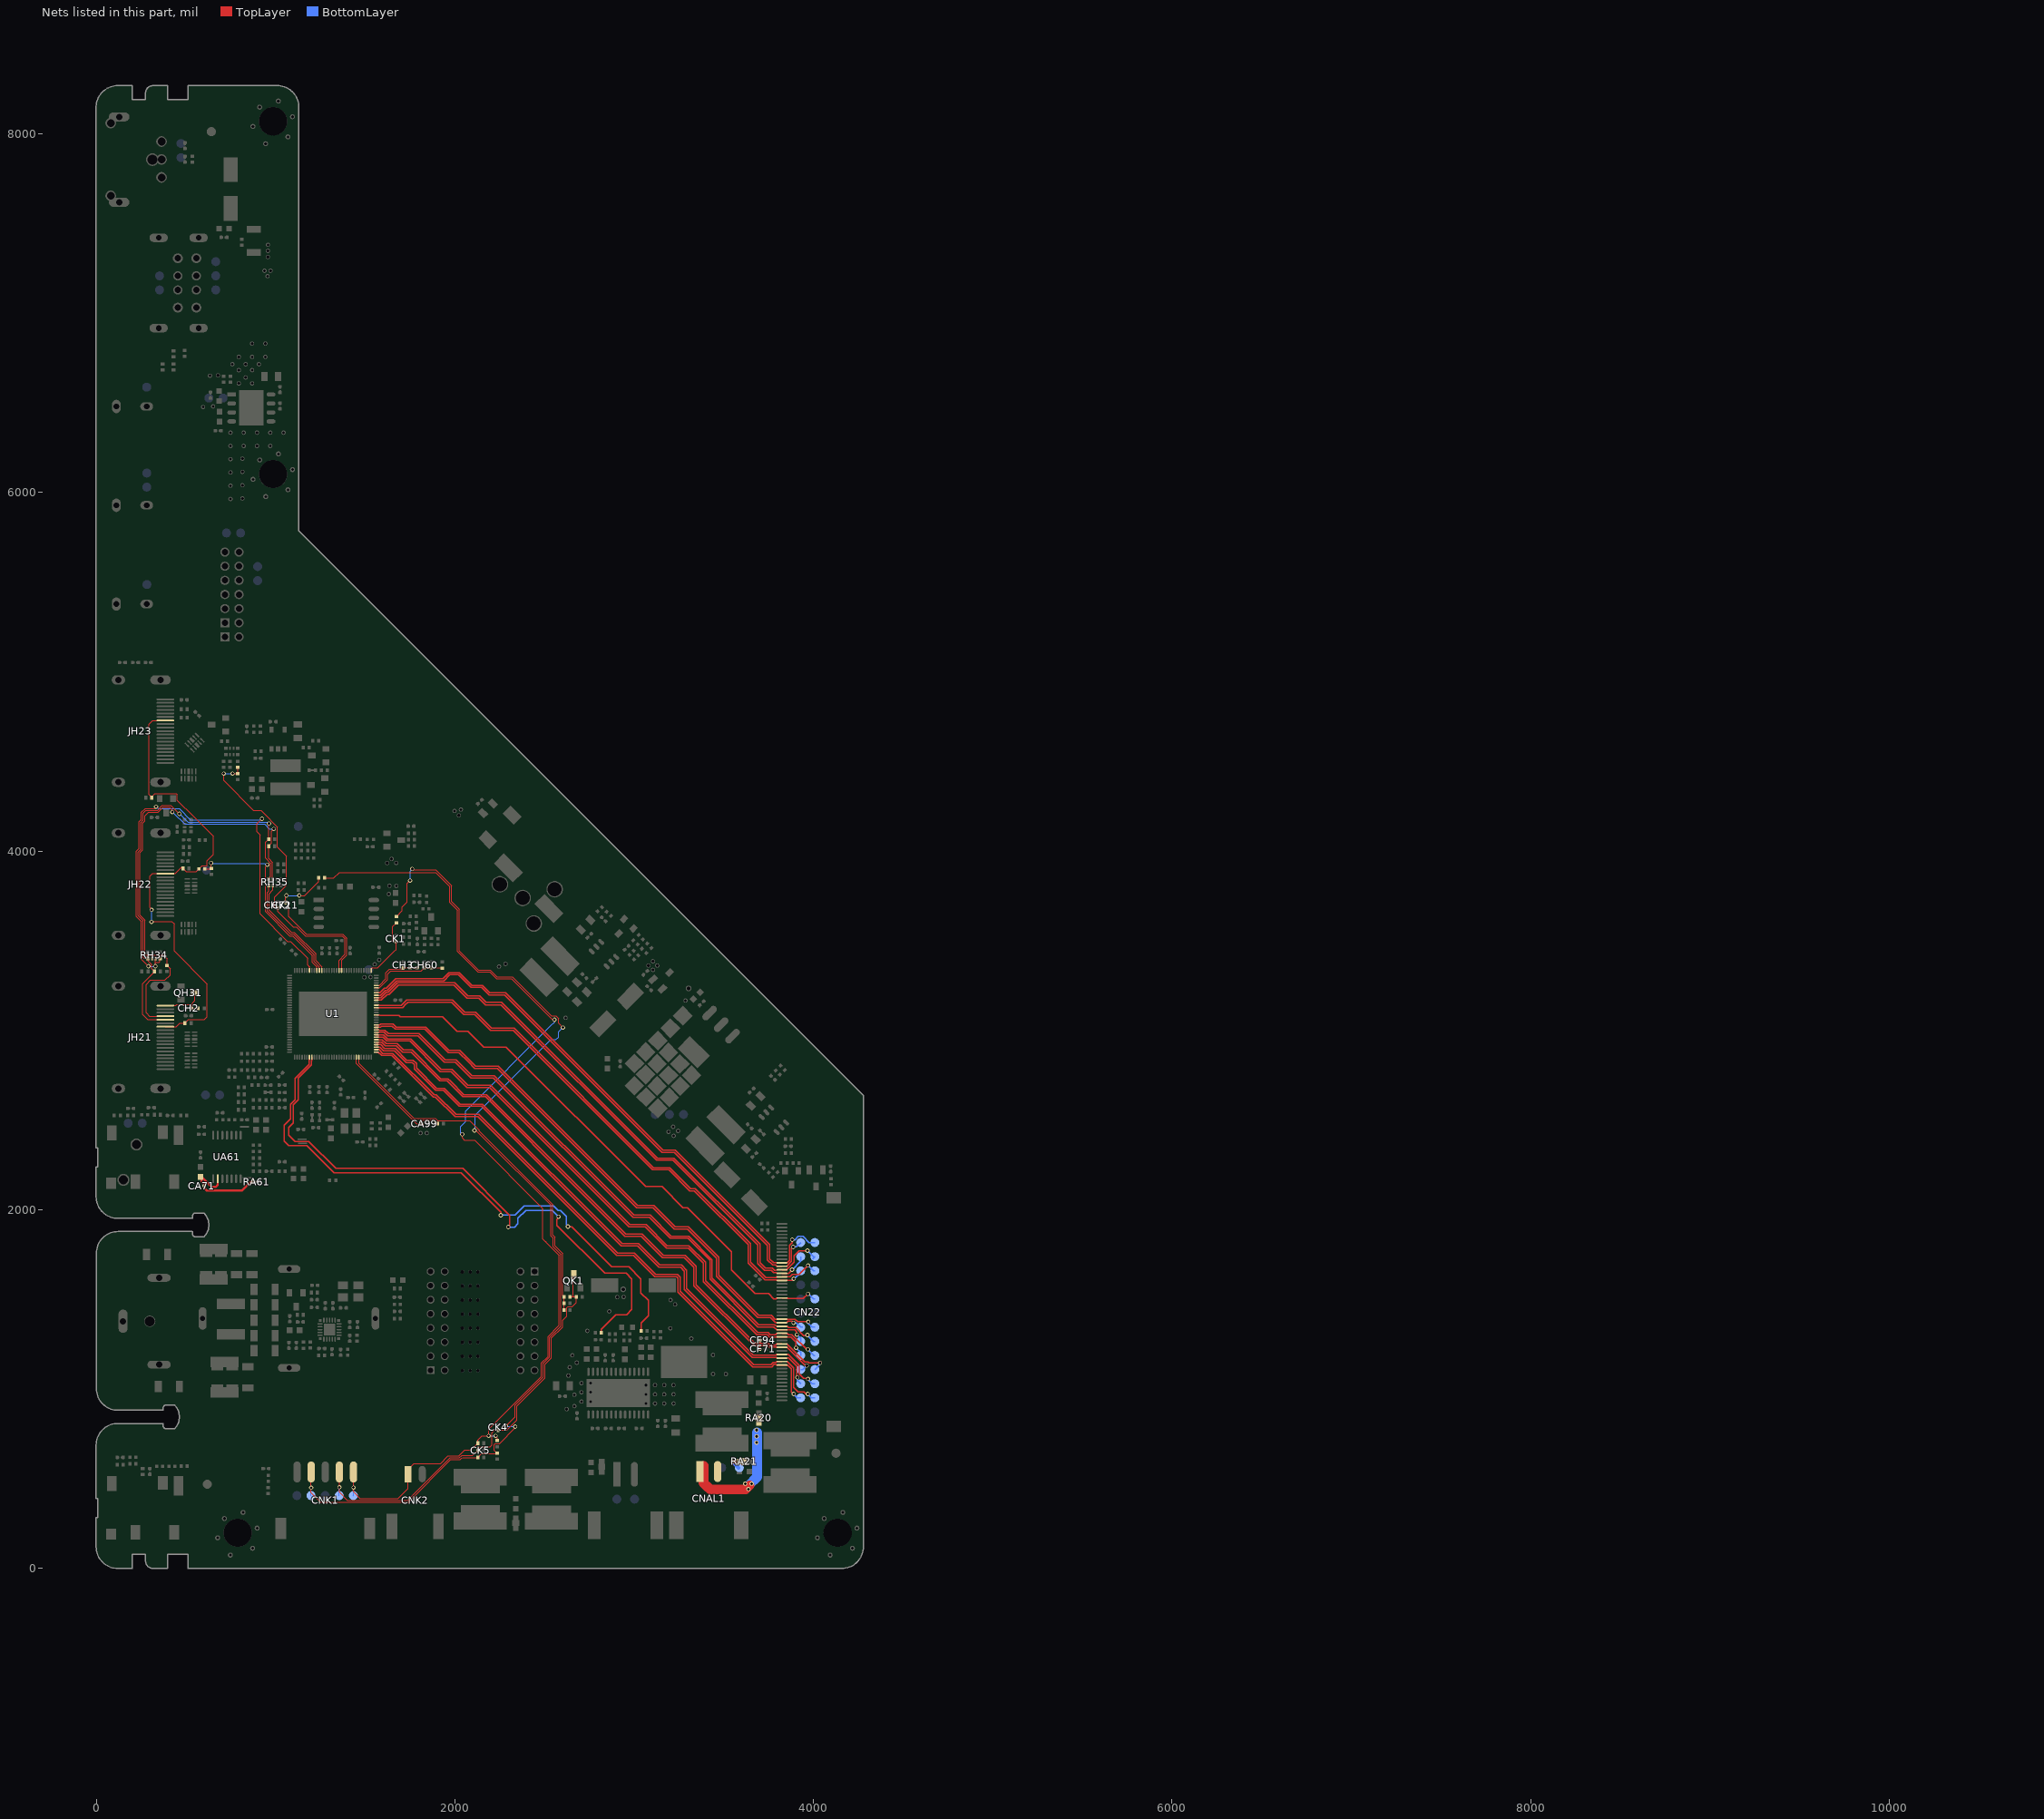
[diagram p0: the nets of this part, all layers, seen from the top]
# Altium PCB MISC105950.PcbDoc (part 11 of 15)
Units mil, origin at the board's own origin, x right, y up, seen from the top; angles counter-clockwise.
Board outline 4280.62 x 8272.76 mil, 2 copper layers (TopLayer, BottomLayer), stack 61.855 mil thick; 541 components, 268 nets, 2324 pads, 1157 vias.

## Via types
v1: diameter 23.62, hole 15.75, TopLayer to BottomLayer, tented both sides, 1087 vias
v2: diameter 23.62, hole 15.75, TopLayer to BottomLayer, 51 vias
v3: diameter 27.56, hole 19.68, TopLayer to BottomLayer, 15 vias
v4: diameter 31.5, hole 19.68, TopLayer to BottomLayer, tented both sides, 4 vias

## Nets (pads, with @x,y where several pads share a name; then routed paths per layer and width w, separated by ;. In a path a pad name is that pad's centre, name@x,y a point inside that pad or via, vN(x,y) a via of type N, cw(c..) or ccw(c..) an arc to the next point about the centre after c; other vN are vias at no path point) (continued)
HDMI_C_HPD_OUT: CH2.1 JH21.19 QH31.C RH33.1 | length 328.2
  TopLayer w5: JH21.19@384.7,3137.25 JH21.19@384.16,3137.8 ; JH21.19@429.3,3137.8 JH21.19@384.16,3137.8 ; 527.65,3142.58 524.92,3142.58 ; QH31.C@549.03,3208 549.03,3166.69 529.23,3146.89 ; RH33.1@566.77,3123 CH2.1@529.23,3123 529.23,3146.89 ; JH21.19@384.16,3137.8 442,3137.8 446.78,3142.58 524.92,3142.58 ; 524.92,3142.58 529.23,3146.89
HDMI_C_HPD_OUT_IC: RH34.2 RH34.4 U1.122 | length 2753
  TopLayer w5: v1(289.26,3357.14) 249.5,3396.9 249.5,3606.45 221.5,3634.45 221.5,3998.62 236.5,4013.62 236.5,4163.19 250.31,4177 250.31,4216.86 271.29,4237.84 v1@327.98,4237.84 ; v1(327.88,3357.14) 327.88,3378 ; RH34.4@330.38,3401.07 327.88,3398.57 327.88,3378 ; RH34.2@354,3401.07 354,3385 347,3378 327.88,3378 ; 913,3994 913,3970 ; v1(922.5,4179.5) 896,4153 896,4108.22 913,4091.22 913,3970 ; U1.122@1185.65,3335.98 U1.122@1187.59,3334.04 1187.59,3352.91 1179.82,3360.68 ; 1185.65,3354.85 1179.82,3360.68 ; 913,3970 913,3648.71 1065.4,3496.31 1082.14,3496.31 1177.66,3400.8 1177.66,3362.84 1179.82,3360.68
  BottomLayer w5: v1(289.26,3357.14) v1(327.88,3357.14) ; v1(331.5,4247.5) 342.64,4236.36 460.95,4236.36 522.81,4174.5 v1@917.5,4174.5
HDMI_C_SCL_IN: DH2.K DH73.K JH21.15 RH34.8 RH35.7 | length 2448.4
  TopLayer w5: DH2.K@322.25,3327.48 DH2.K@323.27,3326.46 ; JH21.15@384.16,3059.06 285.44,3059.06 257.5,3087 257.5,3260.69 DH2.K@323.27,3326.46 ; v1(462,4208) 458.42,4208 412.8,4253.62 365.5,4253.62 339.72,4227.84 275.44,4227.84 260.31,4212.72 260.31,4172.86 246.5,4159.05 246.5,4009.47 231.5,3994.47 231.5,3638.59 259.5,3610.59 259.5,3407 265.43,3401.07 RH34.8@287.07,3401.07 287.07,3386.64 308.57,3365.14 308.57,3349.14 308.57,3343.2 DH2.K@323.27,3328.5 DH2.K@323.27,3326.46 ; RH35.7@960.54,3844.22 960.54,3848.01 971.81,3859.28 971.81,3931.5 943,3960.31 943,4048.47 DH73.K@960.04,4065.5 960.04,4152.04 v1(961.5,4153.5)
  BottomLayer w5: v1(462,4208) 509.81,4160.19 951.81,4160.19 958.5,4153.5 v1(961.5,4153.5)
HDMI_C_SCL_IN_IC: RH35.8 U1.118 | length 607.7
  TopLayer w5: RH35.8@960.54,3808.78 960.54,3777.04 953,3769.5 953,3665.28 1081.81,3536.47 1098.55,3536.47 1213.66,3421.37 1213.66,3383.41 1242.71,3354.36 U1.118@1242.71,3334.04
HDMI_C_SDA_IO: DH3.K DH74.K JH21.16 RH34.6 RH35.5 | length 2559.8
  TopLayer w5: RH34.6@310.69,3401.07 310.69,3418.96 ; JH21.16@384.16,3078.74 295.76,3078.74 276.5,3098 276.5,3254.5 301.16,3279.16 382,3279.16 410.83,3307.98 410.83,3342.91 DH3.K@392.5,3361.23 392.5,3399.36 372.7,3419.16 274.12,3419.16 269.5,3423.78 269.5,3614.74 241.5,3642.74 241.5,3990.33 256.5,4005.33 256.5,4154.9 270.31,4168.72 270.31,4196.98 291.17,4217.84 343.87,4217.84 369.65,4243.62 407.35,4243.62 422.06,4228.92 ; 976.39,4090.89 976.39,4083 ; RH35.5@984.16,3844.22 981.81,3846.56 981.81,3935.64 960.04,3957.42 DH74.K@960.04,4027.5 976.39,4043.86 976.39,4083 ; v1(988.5,4123.5) 976.39,4111.39 976.39,4083
  BottomLayer w5: v1@427.82,4214.49 492.12,4150.19 936.93,4150.19 963.62,4123.5 v1(988.5,4123.5)
  other v1: 422.06,4217.05
HDMI_C_SDA_IO_IC: RH35.6 U1.117 | length 614.9
  TopLayer w5: RH35.6@984.16,3808.78 984.16,3783.39 963,3762.24 963,3669.42 1085.95,3546.47 1102.69,3546.47 1222.66,3426.51 1222.66,3388.56 1256.49,3354.72 U1.117@1256.49,3334.04
HDMI_CEC_IO: DH1.K DH21.K DH70.K JH21.13 JH22.13 JH23.13 RH83.2 | length 2770.9
  TopLayer w5: v1(307,3672) 307,3676.5 297.69,3685.81 297.69,3858.69 313.02,3874.02 JH22.13@384.16,3874.02 438.02,3874.02 474.43,3910.43 DH70.K@481.77,3903.1 500.16,3884.71 555.48,3884.71 RH83.2@570.77,3900 588.11,3917.34 613.34,3917.34 617.38,3921.38 617.38,3946.62 651.16,3980.39 651.16,4081.87 549.52,4183.52 544.28,4188.72 ; v1@307.69,3606.7 419.27,3606.7 432.98,3593 432.98,3441.02 616.59,3257.41 616.59,3075.17 600.73,3059.31 512.81,3059.31 DH1.K@493.5,3040 464.42,3040 444.11,3019.69 JH21.13@384.16,3019.69 ; JH23.13@384.16,4728.35 312.85,4728.35 291.71,4707.21 291.71,4316.02 307.23,4300.5 326.42,4319.69 445.35,4319.69 450.61,4314.43 450.61,4282.39 539.85,4193.15 ; 539.88,4193.15 544.28,4188.76
  BottomLayer w5: v1(306,3604.5) v1@307,3605.5 ; v1@310,3608.5 v1@307,3605.5 ; v1@310,3672 v1(307,3672) v1@307,3605.5
HDMI_CEC_IO_IC: DH4.K RH83.1 U1.119 | length 1126.3
  TopLayer w5: RH83.1@604.36,3900.5 DH4.K@648.66,3900.5 ; v1(638.5,3933) 638.5,3904.73 DH4.K@640,3903.23 ; 943,3897.5 943,3885.5 ; v1(952.5,3923.5) 943,3914 943,3885.5 ; U1.119@1228.93,3334.04 1228.93,3353.99 1204.66,3378.27 1204.66,3416.22 1094.41,3526.47 1077.67,3526.47 943,3661.14 943,3885.5
  BottomLayer w5: v1(638.5,3933) 642,3929.5 938,3929.5 944,3923.5 v1(952.5,3923.5)
HDMIA_DET_IC: CH72.2@1011.5,3681.66 CH72.2@1011.5,3688.55 RH74.1 RH75.1 U1.110 | length 1765.6
  TopLayer w5: v1@700.5,4432.5 v1(709.5,4432.5) 709.5,4392.64 875.16,4226.98 916.63,4226.98 929.61,4214 929.82,4214 1009.86,4133.96 1009.86,4020.99 1060.36,3970.49 1060.36,3810.17 993,3742.81 993,3687 998.34,3681.66 CH72.2@1011.5,3681.66 1011.5,3663.35 1098.38,3576.47 1115.12,3576.47 1165.28,3526.31 1369.79,3526.31 1386.66,3509.44 1386.66,3423.98 1352.95,3390.27 U1.110@1352.95,3334.04 ; v1@757.51,4432.49 RH75.1@787.75,4432.49 ; v1@758.51,4432.49 RH75.1@787.75,4432.49 ; RH75.1@784.5,4436.5 RH75.1@787.75,4433.25 ; RH74.1@787.75,4466.53 RH75.1@787.75,4433.25 ; RH75.1@787.75,4432.49 RH75.1@787.75,4433.25
  BottomLayer w5: v1(709.5,4432.5) v1@757.5,4432.5
  other v1: 758.5,4432.5
HDMIB_DET_IC: CH60.2@1828.5,3347.76 CH60.2@1828.5,3354.65 RH1.1 RH2.1 U1.91 | length 467.9
  TopLayer w5: U1.91@1560.66,3236.56 1577.34,3236.56 1623.94,3283.16 1623.94,3289.05 1623.94,3313.33 1641.11,3330.5 1699.05,3330.5 1699.15,3330.4 1719.85,3330.4 1719.95,3330.5 1723,3330.5 1811.24,3330.5 CH60.2@1828.5,3347.76 ; CH60.2@1829,3348.27 CH60.2@1828.5,3347.76 ; RH2.1@1868.5,3347.77 RH1.1@1928.5,3347.77 ; 1904,3347.76 CH60.2@1828.5,3347.76
HDMIC_DET_IC: CH3.2@1709.5,3346.76 CH3.2@1709.5,3353.65 RH81.1 RH82.1 U1.92 | length 299.6
  TopLayer w5: U1.92@1560.66,3250.34 1576.97,3250.34 1613.94,3287.31 1613.94,3320.3 1634.83,3341.19 1697.04,3341.19 CH3.2@1709.5,3353.65 ; CH3.2@1703.24,3340.5 1711.5,3348.77 RH81.1@1786,3348.77 RH81.1@1784.23,3347
HP_DET_IC: CA99.2@1812.61,2478.5 CA99.2@1819.5,2478.5 RA52.2 U1.58 | length 652
  TopLayer w5: U1.58@1449.41,2849.72 1449.41,2813.71 1784.61,2478.5 CA99.2@1812.61,2478.5 1812.61,2492.61 1817.81,2497.81 1882.96,2497.81 RA52.2@1902.27,2478.5
HP_VDD: CA70.1 CA71.1 RA61.2 RA61.3 UA61.9 | length 546
  TopLayer w12: CA70.1@579.5,2189.19 CA70.1@584.5,2189.19 ; CA70.1@584.5,2183.5 642.5,2125.5 664.5,2125.5 676,2137 UA61.9@676,2171.5 ; CA70.1@584.5,2190 584.5,2157.5 601.86,2140.14 601.86,2118.14 614.54,2105.46 810.38,2105.46 844.96,2140.04 ; 850.26,2145.35 844.96,2140.04 ; RA61.2@875.77,2155 859.92,2155 844.96,2140.04
IR: CNK1.2 DK4.K IR.1 RK6.1 RK25.1 | length 6071
  TopLayer w5: CNK1.2@1197.16,535.5 v1(1197.16,447.88) 1197.16,420.34 1249.12,368.38 1739.45,368.38 1976.29,605.21 2028.87,605.21 2035.51,611.86 2040.15,616.5 DK4.K@2127.27,616.5 2147.96,637.19 RK25.1@2238.96,637.19 ; RK6.1@1673.5,3633.73 1673.5,3634.14 1705.68,3666.32 1705.68,3688.32 1732.91,3715.56 1732.91,3819.41 v1(1748.5,3835) ; v1@1761,3894.5 1893.14,3894.5 1981.5,3806.14 1981.5,3716.92 2023.31,3675.11 2023.31,3443.2 2131.01,3335.5 2196.64,3335.5 2234.33,3297.81 2319.55,3297.81 2538.17,3079.19 2563.31,3079.19 2577.5,3065 2577.5,3039 v1(2601.5,3015) ; v1@2117.31,2441 2155.4,2402.9 2534.31,2023.99 2534.31,1853.1 2547,1840.41 2547,1792.32 2590.5,1748.82 2590.5,1349.04 2528.36,1286.91 2528.36,1176.58 2492.36,1140.58 2492.36,1065.29 2335,907.92 2335,844 v1(2283.5,792.5) ; RK25.1@2231.96,637.19 RK25.1@2235.5,640.73 2234.27,640.73 2218.16,656.84 2218.16,689.23 2223.3,694.37 2248.45,694.37 v1@2335.5,781.42
  BottomLayer w5: IR.1@1196.26,403.88 1197.16,404.78 v1(1197.16,447.88) ; v1@1749,3835 1749,3888.5 v1(1761,3900.5) ; v1@2113.17,2445.67 2113.17,2526.57 2534.28,2947.69 2563.5,2947.69 2577.5,2961.69 2577.5,2991 v1(2601.5,3015) ; v1@2287,789 v1(2335.5,789)
  other v1: 2108.5,2441
IR_IN_IC: CK1.2@1670,3494.26 CK1.2@1670,3501.15 RK6.2 U1.97 | length 410.3
  TopLayer w5: U1.97@1532.08,3334.04 1532.08,3344.58 1536.5,3349 1569.1,3349 1661.49,3441.38 1670.47,3450.36 CK1.2@1670.47,3497.8 ; 1652.66,3514.36 1652.66,3529 ; 1652.66,3553.93 1652.66,3529 ; CK1.2@1668.75,3498.26 CK1.2@1670,3498.26 ; CK1.2@1670,3494.26 1657.24,3494.26 1652.66,3498.84 1652.66,3529 ; RK6.2@1673.5,3600.27 1652.66,3579.43 1652.66,3529
K0/AD: CNK1.5 CNK2.1 DK70.K KEY.1 RK2.1 RK23.2 | length 6035.5
  TopLayer w5: RK23.2@1271.73,3850 1323.5,3850 1354.5,3881 1892.5,3881 1971.5,3802 1971.5,3712.78 2013.31,3670.97 2013.31,3439.06 2126.87,3325.5 2167,3325.5 ; CNK1.5@1433.25,535.38 v1(1433.25,449.13) 1433.25,424.75 1469.62,388.38 1681.73,388.38 1737.84,444.48 CNK2.1@1737.84,496.04 ; CNK2.1@1737.84,523.69 1737.84,551.34 1770,583.5 1919,583.5 1960.71,625.21 2020.58,625.21 2053.87,658.5 2088.77,658.5 DK70.K@2127.27,697 2127.27,714.33 2150.44,737.5 v1(2187.5,737.5) 2187.5,774.56 2482.36,1069.43 2482.36,1144.72 2518.36,1180.72 2518.36,1291.05 2580.5,1353.18 2580.5,1744.68 2513.09,1812.09 ; v1(2040,2419.5) 2040,2398.5 2052.5,2386 2108.67,2386 2489.31,2005.35 2489.31,1835.87 2513.09,1812.09 ; 2134.22,3325.5 2167,3325.5 ; v1(2226.5,737.5) 2226.5,733 2235.5,724 RK2.1@2235.5,710.73 ; 2503.2,1821.98 2513.09,1812.09 ; v1(2554.22,3058.57) 2553,3057.35 2553,3050.22 2315.4,3287.81 2230.19,3287.81 2192.5,3325.5 2167,3325.5
  BottomLayer w5: KEY.1@1432.48,403.88 1433.25,404.65 v1(1433.25,449.13) ; v1(2040,2419.5) 2032,2427.5 2032,2463.86 2058.17,2490.02 2058.17,2549.35 2535,3026.19 ; v1(2187.5,737.5) v1(2226.5,737.5) ; 2541,3032.19 2535,3026.19 ; v1(2554.22,3058.57) 2554.22,3045.41 2535,3026.19
KEY_IN_IC: CK11.1 RK23.1 U1.109 | length 953.2
  TopLayer w5: v1(1059.5,3752) 1053.5,3746 CK11.1@1053.5,3716.63 ; v1@1130.07,3754 1128.5,3754 v1(1130.5,3752) 1160.3,3752 1238.27,3829.97 RK23.1@1238.27,3850 ; U1.109@1366.73,3334.04 1368.01,3335.31 1368.01,3391.19 1396.66,3419.84 1396.66,3513.59 1373.93,3536.31 1169.42,3536.31 1117.09,3588.64 1116.88,3588.64 1071,3634.52 1071,3711.5 1067.37,3715.13 CK11.1@1055,3715.13 ; CK11.1@1053.5,3716.63 CK11.1@1053.5,3715.13 CK11.1@1055,3715.13 ; CK11.1@1053.5,3716.63 CK11.1@1055,3715.13
  BottomLayer w5: v1(1059.5,3752) 1086,3752 ; 1098.5,3752 1086,3752 ; v1(1130.5,3752) 1086,3752
LED_R_OUT: CK4.2@2240,767.76 CK4.2@2240,774.65 CK5.2@2126.27,656.5 CK5.2@2133.16,656.5 CNK1.4 LED.1 QK1.C RK10.1 RK14.2 | length 2398
  TopLayer w5: CNK1.4@1354.64,535.5 v1(1354.64,450.24) 1354.64,422.36 1398.62,378.38 1735.31,378.38 1972.14,615.21 2024.72,615.21 2037.4,627.9 2097.66,627.9 CK5.2@2126.27,656.5 2126.27,670.77 2131.31,675.81 2195.24,675.81 2206.81,687.39 2206.81,753.81 2223,770 2289.19,770 2345,825.81 2345,903.78 2502.36,1061.14 2502.36,1136.44 2538.36,1172.44 2538.36,1282.76 2600.5,1344.9 2600.5,1381 2624.37,1404.87 2624.37,1452.95 2630.58,1459.16 2653.2,1459.16 2675.77,1481.73 RK10.1@2675.77,1512.5 2659,1512.5 ; RK14.2@2641.23,1512.5 2659,1512.5 ; QK1.C@2662,1638.03 2659,1635.03 2659,1512.5
  BottomLayer w5: LED.1@1353.74,403.88 v1@1353.74,449.34
LED_R_OUT_IC: RK13.1 RK14.1 RK15.1 U1.59 | length 2060.5
  TopLayer w5: U1.59@1463.19,2849.72 1463.19,2814.07 1769.44,2507.81 1889.53,2507.81 1901.5,2495.84 2080.97,2495.84 2135.31,2441.5 2135.31,2437.14 2544.31,2028.14 2544.31,1858.65 2557,1845.96 2557,1796.47 2600.5,1752.97 2600.5,1519.77 RK14.1@2607.27,1513 ; RK13.1@2607.77,1440.5 RK13.1@2607.27,1440 RK14.1@2607.27,1513 ; RK14.1@2607.77,1512.5 RK14.1@2607.27,1513
LINE_L_OUT_IC: RA3.1 U1.39 | length 3231.6
  TopLayer w7: 1185.82,2830 1185.82,2826 ; U1.39@1187.59,2849.72 1187.59,2835.91 1185.82,2834.13 1185.82,2826 ; v1(2255.15,1968.38) 2255.15,1983.55 2033.69,2205 1325.45,2205 1174.11,2356.34 1072.43,2356.34 1047.69,2381.09 1047.69,2471.19 1082,2505.5 1082,2587 1107,2612 1107,2731.94 1185.82,2810.76 1185.82,2826 ; v1(2629.62,1904.36) 2649.87,1904.36 2873.72,1680.5 2968.75,1680.5 3037,1612.25 3037,1534.56 3078.95,1492.6 3078.95,1408.5 3037.27,1366.81 RA3.1@3037.27,1322
  BottomLayer w7: v1(2255.15,1968.38) 2334.24,1968.38 2385.16,2019.31 2551.13,2019.31 2575.94,1994.5 2588.97,1994.5 2621.31,1962.16 v1@2621.31,1912.67
LINE_R_OUT_IC: RA14.1 U1.40 | length 3338.8
  TopLayer w7: 1134.03,2380.34 1155.5,2380.34 ; U1.40@1200.43,2848.77 U1.40@1201.37,2849.72 1201.37,2832.71 1197.82,2829.16 1197.82,2805.79 1124.5,2732.47 1124.5,2612.53 1096.5,2584.53 1096.5,2482.72 1072.19,2458.41 1072.19,2414.62 1106.46,2380.34 1155.5,2380.34 ; v1@2297.5,1902 v1(2297,1902) 2305.5,1910.5 2305.5,1967.13 2043.63,2229 1335.39,2229 1184.05,2380.34 1155.5,2380.34 ; v1@2577,1953.69 2568.31,1945 2568.31,1911.02 2834.83,1644.5 2953.84,1644.5 2986,1612.34 2986,1442 2956.5,1412.5 2897,1412.5 2815.76,1331.26 RA14.1@2815.76,1312.23
  BottomLayer w7: v1@2301.79,1902 2332.03,1902 2351,1920.97 2351,1951.21 2395.1,1995.31 2541.19,1995.31 v1(2577,1959.5)
LOUT+: CNAL1.1 LOUT+.1 pad.VIA5@3618.4,470.2 pad.VIA5@3636.5,439.9 pad.VIA5@3654.5,470.5 pad.VIA5@3681.8,699.2 pad.VIA5@3682,770 pad.VIA5@3682.5,734.3 RA20.2 RA20.3 | length 691.5
  TopLayer w55: 3387.5,570 3387,569.5 3387,474 3411,450 3423,438 3620.31,438 3643.28,460.97
  BottomLayer w55: 3638,461 3684.19,507.19 3684.19,756.5
LOUT-: CNAL1.2 LOUT-.1 RA21.2 RA21.3 | length 85.2
  TopLayer w20: v1(3546.5,594) RA21.2@3582.72,594
  BottomLayer w20: v1(3546.5,594) LOUT-.1@3581.13,559.37
LVDS_E0N_IC: CN22.24 E0N.1 U1.76 | length 3212.3
  TopLayer w7: U1.76@1560.66,3029.87 1561.61,3030.82 1581.8,3030.82 1586.19,3035.21 1653.49,3035.21 1670.69,3018 1836.67,3018 1966.49,2888.18 2027.11,2888.18 2115.59,2799.69 2240.93,2799.69 3019.12,2021.5 3110,2021.5 3227.45,1904.05 3300.78,1904.05 3469.95,1734.88 3469.95,1632.37 3692.8,1409.53 3764.35,1409.53 3785.9,1387.98 CN22.24@3823.43,1387.98 3895,1387.98 3896.24,1387.98 3910.22,1374 v1(3970,1374)
  BottomLayer w7: v1@3965.5,1369.5 3991.8,1343.2 E0N.1@4007.24,1343.2
LVDS_E0P_IC: CN22.23 E0P.1 U1.75 | length 3115.5
  TopLayer w7: U1.75@1560.66,3016.09 1584.05,3016.09 1591.16,3023.21 1648.52,3023.21 1665.72,3006 1831.7,3006 1961.52,2876.18 2022.14,2876.18 2073.6,2824.71 2110.62,2787.69 2235.96,2787.69 3014.15,2009.5 3105.03,2009.5 3222.48,1892.05 3295.81,1892.05 3457.95,1729.91 3457.95,1627.4 3687.83,1397.53 3759.38,1397.53 3788.61,1368.3 CN22.23@3823.43,1368.3 ; CN22.23@3850.82,1368.3 3858.5,1375.98 3879.52,1375.98 v1(3888,1367.5)
  BottomLayer w7: v1(3888,1367.5) 3904.2,1367.5 E0P.1@3928.5,1343.2 E0P.1@3938.3,1343.2
LVDS_E1N_IC: CN22.22 E1N.1 U1.74 | length 3191.8
  TopLayer w7: U1.74@1560.66,3002.31 1575.22,3002.31 ; 1577,3000.53 1608.97,3000.53 1627.5,2982 1797.71,2982 1944.53,2835.18 2005.15,2835.18 2012.92,2827.42 2093.64,2746.69 2218.98,2746.69 2997.17,1968.5 3088.05,1968.5 3205.5,1851.05 3302.87,1851.05 3433.95,1719.97 3433.95,1617.46 3694.85,1356.57 3783.37,1356.57 3791.33,1348.61 ; CN22.22@3823.43,1348.61 3854.39,1348.61 3862.07,1340.93 3901.07,1340.93 3945,1297 v1@3964,1297
  BottomLayer w7: v1@3964,1297 3967,1297 3999.54,1264.46 E1N.1@4007.24,1264.46
  other v1: 3966,1300
LVDS_E1P_IC: CN22.21 E1P.1 U1.73 | length 3162.5
  TopLayer w7: U1.73@1560.66,2988.53 1603.47,2988.53 1622.5,2969.5 1793.24,2969.5 1939.56,2823.18 2000.18,2823.18 2088.67,2734.69 2214.01,2734.69 2992.2,1956.5 3083.08,1956.5 3200.53,1839.05 3297.9,1839.05 3421.95,1714.99 3421.95,1612.49 3689.88,1344.57 3778.4,1344.57 3794.04,1328.93 CN22.21@3823.43,1328.93 3895.57,1328.93 3907,1317.5 v1(3907,1302) v1@3905,1302
  BottomLayer w7: v1(3907,1302) 3928.5,1280.5 E1P.1@3928.5,1264.46
LVDS_E2N_IC: CN22.20 E2N.1 U1.72 | length 3222
  TopLayer w7: U1.72@1560.66,2974.75 1575.72,2974.75 ; 1577.53,2972.97 1602.06,2972.97 1622.53,2952.5 1752.26,2952.5 1922.58,2782.18 1983.2,2782.18 2071.69,2693.69 2197.03,2693.69 2975.21,1915.5 3066.09,1915.5 3183.55,1798.05 3304.96,1798.05 3397.95,1705.05 3397.95,1602.55 3687.89,1312.61 3746.85,1312.61 3757.9,1301.56 3786.24,1301.56 CN22.20@3793.93,1309.24 ; CN22.20@3823.43,1309.24 3853.82,1309.24 3861.5,1301.56 3878.44,1301.56 v1@3966,1214
  BottomLayer w7: v1@3966,1214 3973,1214 4001.28,1185.72 E2N.1@4007.24,1185.72
  other v1: 3968,1220
LVDS_E2P_IC: CN22.19 E2P.1 U1.71 | length 3191.8
  TopLayer w7: U1.71@1560.66,2960.97 1597.09,2960.97 1617.56,2940.5 1747.29,2940.5 1917.61,2770.18 1978.23,2770.18 2028.95,2719.45 2066.72,2681.69 2192.06,2681.69 2970.24,1903.5 3061.12,1903.5 3180.25,1784.37 3301.67,1784.37 3385.95,1700.08 3385.95,1597.58 3682.92,1300.61 3741.88,1300.61 3752.93,1289.56 CN22.19@3823.43,1289.56 3873.47,1289.56 3902.5,1260.53 v1(3902.5,1228.5)
  BottomLayer w7: v1(3902.5,1228.5) 3928.5,1202.5 E2P.1@3928.5,1185.72
LVDS_E3N_IC: CN22.14 E3N.1 U1.68 | length 3339.7
  TopLayer w7: U1.68@1560.66,2919.63 1584.87,2919.63 1606.5,2898 1665.97,2898 1731.16,2832.81 1765.88,2832.81 1784.81,2813.88 1784.81,2789.43 1898.06,2676.18 1939.29,2676.18 1957.99,2657.49 2027.78,2587.69 2153.12,2587.69 2931.31,1809.5 3022.19,1809.5 3141.32,1690.37 3262.73,1690.37 3291.95,1661.15 3291.95,1558.64 3663.66,1186.94 3790,1186.94 3794.19,1191.13 CN22.14@3823.43,1191.13 3857.84,1191.13 3918,1130.97 3918,1084 3945,1057 3961,1057 3966.5,1051.5 v1@3971,1056
  BottomLayer w7: v1@3968.5,1051.5 3991.76,1028.24 E3N.1@4007.24,1028.24
  other v1: 3969,1055
LVDS_E3P_IC: CN22.13 E3P.1 U1.67 | length 3264
  TopLayer w7: U1.67@1560.66,2905.85 1581.68,2905.85 1601.53,2886 1661,2886 1726.19,2820.81 1760.91,2820.81 1772.81,2808.91 1772.81,2784.46 1893.09,2664.18 1934.32,2664.18 2022.81,2575.69 2148.15,2575.69 2926.34,1797.5 3017.22,1797.5 3136.35,1678.37 3257.76,1678.37 3279.95,1656.18 3279.95,1553.67 3658.69,1174.94 3791.5,1174.94 3794.99,1171.45 CN22.13@3823.43,1171.45 3860.55,1171.45 3906,1126 3906,1067 v1(3909.5,1063.5)
  BottomLayer w7: v1(3909.5,1063.5) 3909.5,1047.24 E3P.1@3928.5,1028.24
LVDS_E4N_IC: CN22.12 E4N.1 U1.66 | length 3345.6
  TopLayer w7: U1.66@1560.66,2892.07 1574.47,2892.07 1595.55,2871 1652.33,2871 1883.15,2640.18 1895.46,2640.18 2004.8,2530.84 2133.13,2530.84 2907.47,1756.5 3000.23,1756.5 3119.36,1637.37 3240.78,1637.37 3255.95,1622.19 3255.95,1543.73 3665.75,1133.94 3762.04,1133.94 3775.67,1147.57 3790,1147.57 3794.19,1151.76 CN22.12@3823.43,1151.76 ; 3854.21,1151.76 3889,1116.97 3889,1007.5 3913,983.5 3947.5,983.5 3960.5,970.5 v1(3967.5,970.5)
  BottomLayer w7: v1(3967.5,970.5) 3967.5,970 3988,949.5 E4N.1@4007.24,949.5
LVDS_E4P_IC: CN22.11 E4P.1 U1.65 | length 3299.9
  TopLayer w7: U1.65@1560.66,2878.29 1571.28,2878.29 1590.58,2859 1647.36,2859 1878.18,2628.18 1890.49,2628.18 1999.83,2518.84 2128.16,2518.84 2902.5,1744.5 2995.26,1744.5 3114.39,1625.37 3235.81,1625.37 3243.95,1617.22 3243.95,1538.76 3660.78,1121.94 3767.01,1121.94 3780.64,1135.57 3790,1135.57 3793.49,1132.08 CN22.11@3823.43,1132.08 3856.92,1132.08 3877,1112 3877,982.5 v1(3889,970.5)
  BottomLayer w7: v1(3889,970.5) 3910,949.5 E4P.1@3928.5,949.5
LVDS_ECKN_IC: CF94.2@3699.77,1270.18 CF94.2@3706.66,1270.18 CN22.17 ECKN.1 U1.70 | length 3325.7
  TopLayer w7: U1.70@1560.66,2947.19 1593.9,2947.19 1615.09,2926 1677,2926 1712.94,2890.06 1759.54,2890.06 1920.43,2729.18 1961.25,2729.18 1975.43,2715 2049.73,2640.69 2175.07,2640.69 2953.26,1862.5 3044.14,1862.5 3163.27,1743.37 3284.68,1743.37 3344.95,1683.1 3344.95,1580.6 3673.72,1251.84 3747.98,1251.84 3755.94,1243.88 3787.89,1243.88 3794.19,1250.19 CN22.17@3823.43,1250.19 ; 3701.26,1253.1 CF94.2@3701.26,1270.18 ; CN22.17@3851.31,1250.19 3952.19,1149.31 3970.41,1149.31 3975.81,1143.91 4035.91,1143.91 v1(4036,1144)
  BottomLayer w7: ECKN.1@4007.24,1106.98 4036,1135.74 v1(4036,1144)
LVDS_ECKP_IC: CF71.2@3699.77,1221.48 CF71.2@3706.66,1221.48 CN22.16 ECKP.1 U1.69 | length 3268
  TopLayer w7: U1.69@1560.66,2933.41 1590.71,2933.41 1610.12,2914 1672.03,2914 1707.97,2878.06 1754.57,2878.06 1915.46,2717.18 1956.28,2717.18 2044.76,2628.69 2170.1,2628.69 2695.4,2103.4 2948.29,1850.5 3039.17,1850.5 3158.3,1731.37 3279.71,1731.37 3332.95,1678.13 3332.95,1575.63 3668.75,1239.84 3743.01,1239.84 3750.97,1231.88 3792.82,1231.88 3794.19,1230.5 CN22.16@3823.43,1230.5 3854.03,1230.5 3955.53,1129 v1(3962,1129) ; CF71.2@3699.77,1221.48 3699.77,1238.06
  BottomLayer w7: ECKP.1@3928.5,1106.98 3939.98,1106.98 v1(3962,1129)
LVDS_O0N_IC: CN22.40 O0N.1 U1.89 | length 3319.1
  TopLayer w7: U1.89@1560.66,3209 1579.48,3209 1605.15,3234.68 1615.46,3234.68 1668.78,3288 1932.98,3288 1966.48,3321.5 2023.51,3321.5 2094.51,3250.5 2152.97,3250.5 2194.28,3209.19 2281.15,3209.19 2827.51,2662.84 3159.34,2331 3227.38,2331 3754.5,1803.88 3754.5,1724.89 3776.44,1702.94 CN22.40@3823.43,1702.94 ; CN22.40@3851.97,1702.94 3865.01,1715.99 3865.01,1799.01 3881,1815 v1(3881,1831)
  BottomLayer w7: v1@3882,1830 v1(3881,1831) 3896.48,1831 3914.62,1849.14 3942.38,1849.14 3975.88,1815.64 O0N.1@4007.24,1815.64 O0N.1@4003.36,1815.64
LVDS_O0P_IC: CN22.39 O0P.1 U1.88 | length 3205.3
  TopLayer w7: U1.88@1560.66,3195.22 1582.67,3195.22 1610.12,3222.68 1620.43,3222.68 1673.75,3276 1937.95,3276 1971.45,3309.5 2018.54,3309.5 2089.54,3238.5 2148,3238.5 2189.31,3197.19 2276.18,3197.19 2815.51,2657.87 3154.37,2319 3222.41,2319 3742.5,1798.91 3742.5,1719.92 3771.47,1690.94 3787.44,1690.94 3795.12,1683.26 CN22.39@3823.43,1683.26 ; CN22.39@3850.26,1683.26 3877.01,1710.01 3877.01,1756.74 3877.01,1781.01 3886,1790 v1(3886,1791)
  BottomLayer w7: v1(3886,1791) 3903.5,1791 3928.14,1815.64 O0P.1@3928.5,1815.64
LVDS_O1N_IC: CN22.38 O1N.1 U1.87 | length 3277.7
  TopLayer w7: U1.87@1548.5,3180.5 U1.87@1549.45,3181.44 ; U1.87@1560.66,3180.5 1584.91,3180.5 1615.09,3210.68 1626.18,3210.68 1679.5,3264 1998.5,3264 2070.49,3192.01 2136.51,3192.01 2172.33,3156.19 2259.2,3156.19 2408,3007.39 3128.89,2286.5 3220.97,2286.5 3700.95,1806.52 3700.95,1704.01 3732.34,1672.63 3769.25,1672.63 3782.5,1659.38 3790,1659.38 CN22.38@3794.19,1663.57 ; CN22.38@3823.43,1663.57 3848.32,1663.57 3890,1705.25 3890,1741 3919,1770 v1@3963,1770
  BottomLayer w7: v1@3966,1773 3966,1767 3969,1767 3999.1,1736.9 O1N.1@4007.24,1736.9 O1N.1@3994.84,1724.5
  other v1: 3966,1771
LVDS_O1P_IC: CN22.37 O1P.1 U1.86 | length 3166.8
  TopLayer w7: U1.86@1560.66,3167.66 1589.05,3167.66 1620.06,3198.68 1631.15,3198.68 1684.47,3252 1993.53,3252 2065.52,3180.01 2131.54,3180.01 2170.37,3141.18 2257.24,3141.18 3123.92,2274.5 3216,2274.5 3688.95,1801.55 3688.95,1699.04 3727.37,1660.63 3764.28,1660.63 3777.53,1647.38 3791.5,1647.38 CN22.37@3794.99,1643.89 ; CN22.37@3823.43,1643.89 3859.89,1643.89 v1(3880,1664)
  BottomLayer w7: v1(3880,1664) 3928.5,1712.5 O1P.1@3928.5,1734 ; O1P.1@3928.5,1720.5 O1P.1@3928.5,1734 ; O1P.1@3928.5,1736.9 O1P.1@3928.5,1734
LVDS_O2N_IC: CN22.36 O2N.1 U1.84 | length 3239.5
  TopLayer w7: U1.84@1560.66,3140.11 1574.72,3140.11 ; 1576.5,3138.33 1699.33,3138.33 1729.27,3168.27 1986.21,3168.27 2054.3,3100.18 2114.92,3100.18 2203.41,3011.69 2328.75,3011.69 3106.93,2233.5 3197.81,2233.5 3315.27,2116.05 3340.51,2116.05 3647.95,1808.61 3647.95,1706.1 3734.05,1620.01 3790,1620.01 CN22.36@3794.19,1624.2 ; 3854.31,1624.2 CN22.36@3823.43,1624.2 ; 3862.2,1624.2 CN22.36@3823.43,1624.2 ; v1(3969,1688) 3918,1637 3881,1637 3868.2,1624.2 CN22.36@3823.43,1624.2
  BottomLayer w7: v1(3969,1688) 3998.84,1658.16 O2N.1@4007.24,1658.16
LVDS_O2P_IC: CN22.35 O2P.1 U1.83 | length 3131.1
  TopLayer w7: U1.83@1560.66,3126.33 1706.33,3126.33 1725.16,3145.16 ; 1731.77,3151.77 1725.16,3145.16 ; 1985.74,3151.77 1993.38,3144.13 ; v1@3892,1612 3884.52,1604.52 CN22.35@3823.43,1604.52 3794.99,1604.52 3791.5,1608.01 3729.08,1608.01 3635.95,1701.13 3635.95,1803.64 3335.54,2104.05 3310.29,2104.05 3192.84,2221.5 3101.96,2221.5 2323.78,2999.69 2198.44,2999.69 2109.95,3088.18 2049.33,3088.18 1993.38,3144.13 ; 1725.16,3145.16 1736.27,3156.27 1981.24,3156.27 1993.38,3144.13
  BottomLayer w7: v1@3892,1612 3928.5,1648.5 O2P.1@3928.5,1658.16
  other v1: 3889,1614
LVDS_O3N_IC: CN22.30 O3N.1 U1.80 | length 3159.5
  TopLayer w7: U1.80@1560.66,3084.99 1577.72,3084.99 ; 1579.5,3083.21 1687.47,3083.21 1695.18,3075.5 1929.07,3075.5 2010.39,2994.18 2071.01,2994.18 2159.5,2905.69 2284.84,2905.69 3063.03,2127.5 3153.91,2127.5 3271.36,2010.05 3296.61,2010.05 3541.95,1764.7 3541.95,1662.2 3673.14,1531.01 3749.23,1531.01 3778.34,1501.9 3790,1501.9 CN22.30@3794.19,1506.09 ; CN22.30@3823.43,1506.09 3855.41,1506.09 3858.81,1502.69 3942.69,1502.69 v1(3969,1529)
  BottomLayer w7: v1(3969,1529) 3969,1523.68 3977.32,1523.68 4000.32,1500.68 O3N.1@4007.24,1500.68